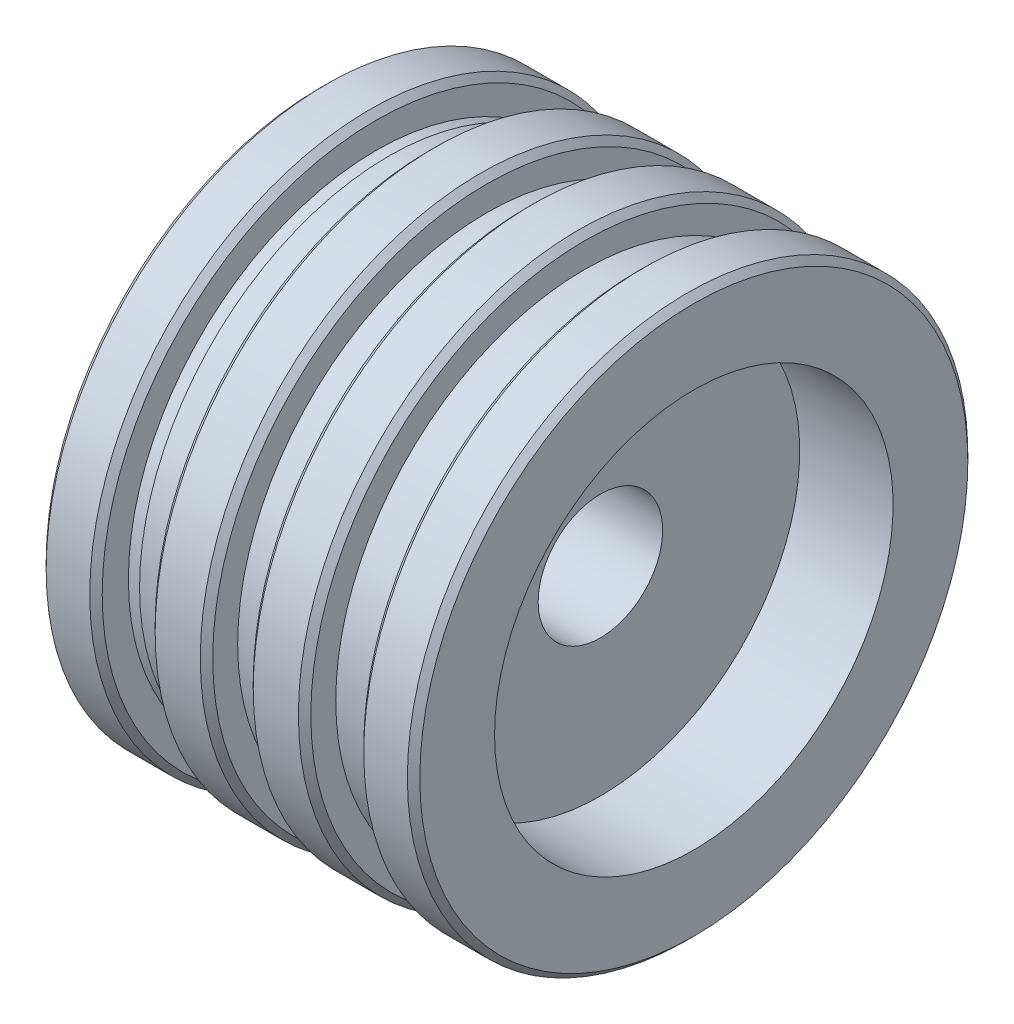
SolidWorks part; units mm, degrees
ref_plane "前视基准面" through (0, 0, 0) normal (0, 0, 1) x (1, 0, 0)
ref_plane "上视基准面" through (0, 0, 0) normal (0, 1, 0) x (1, 0, 0)
ref_plane "右视基准面" through (0, 0, 0) normal (1, 0, 0) x (0, 0, -1)
other "Configuration Table"
sketch "草图1" plane through (0, 0, 0) normal (0, 1, 0) x (1, 0, 0)
  line L0 (0, 0) -> (40.8247, 0) construction
  line L1 (0, 16) -> (0, 45)
  line L2 (0, 45) -> (9, 45)
  line L3 (9, 45) -> (9, 39.8)
  line L5 (17.5, 40) -> (17.5, 45)
  line L6 (17.5, 45) -> (26.75, 45)
  line L7 (26.75, 45) -> (26.75, 40)
  line L8 (26.75, 40) -> (33.25, 40)
  line L9 (33.25, 40) -> (33.25, 45)
  line L10 (33.25, 45) -> (42.5, 45)
  line L11 (42.5, 45) -> (42.5, 40)
  line L13 (51, 39.8) -> (51, 45)
  line L14 (51, 45) -> (60, 45)
  line L15 (60, 45) -> (60, 32)
  line L16 (60, 32) -> (45, 32)
  line L17 (45, 32) -> (45, 10)
  line L18 (45, 10) -> (30, 10)
  line L19 (30, 10) -> (30, 16)
  line L20 (30, 16) -> (0, 16)
  line L21 (9, 39.8) -> (11, 39.8)
  line L22 (11, 39.8) -> (11, 40)
  line L23 (11, 40) -> (17.5, 40)
  line L24 (51, 39.8) -> (49, 39.8)
  line L25 (49, 39.8) -> (49, 40)
  line L26 (49, 40) -> (42.5, 40)
  dimension "D1" = 90
  dimension "D2" = 32
  dimension "D3" = 64
  dimension "D4" = 20
  dimension "D5" = 9
  dimension "D6" = 2
  dimension "D7" = 0.2
  dimension "D8" = 8.5
  dimension "D9" = 9.25
  dimension "D10" = 6.5
  dimension "D11" = 2
  dimension "D12" = 0.2
  dimension "D13" = 9.25
  dimension "D14" = 8.5
  dimension "D15" = 60
  dimension "D16" = 80
  dimension "D17" = 30
  dimension "D18" = 15
revolve "旋转1" add sketch "草图1" angle 360 about L0
chamfer "倒角1" distance 1 angle 45 8 edges at (60, 0, 45) (51, 0, 45) (42.5, 0, 45) (33.25, 0, 45) (26.75, 0, 45) (17.5, 0, 45) (9, 0, 45) (0, 0, 45)
